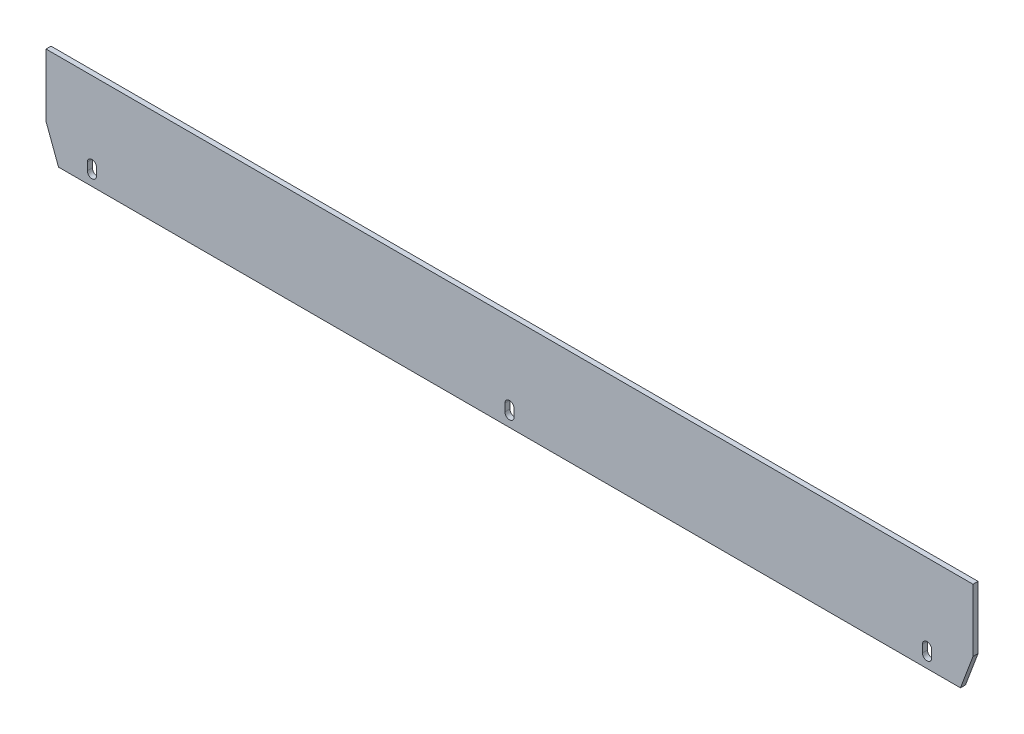
SolidWorks part; units mm, degrees
material "1023 碳钢板 (SS)"
ref_plane "Front Plane" through (0, 0, 0) normal (0, 0, 1) x (1, 0, 0)
ref_plane "Top Plane" through (0, 0, 0) normal (0, 1, 0) x (1, 0, 0)
ref_plane "Right Plane" through (0, 0, 0) normal (1, 0, 0) x (0, 0, -1)
sketch "Sketch1" plane through (0, 0, 0) normal (0, 0, 1) x (1, 0, 0)
  line L1 (555, -57.5) -> (-555, -57.5)
  line L2 (555, -57.5) -> (555, 57.5)
  line L3 (555, 57.5) -> (-555, 57.5)
  line L4 (-555, -57.5) -> (-555, 57.5)
  line L5 (555, -57.5) -> (-555, 57.5) construction
  line L6 (555, 57.5) -> (-555, -57.5) construction
  point P0 (0, 0)
  dimension "D1" = 1110
  dimension "D2" = 115
extrude "Boss-Extrude1" add sketch "Sketch1" along normal blind 6
sketch "Sketch2" plane through (0, 0, 6) normal (0, 0, 1) x (1, 0, 0)
  line L0 (-500, -35) -> (-500, -44) construction
  line L1 (-494.5, -35) -> (-494.5, -44)
  line L2 (-505.5, -35) -> (-505.5, -44)
  line L3 (0, -35) -> (0, -44) construction
  line L4 (5.5, -35) -> (5.5, -44)
  line L5 (-5.5, -35) -> (-5.5, -44)
  line L6 (500, -44) -> (500, -35) construction
  line L7 (494.5, -44) -> (494.5, -35)
  line L8 (505.5, -44) -> (505.5, -35)
  line L9 (-555, -57.5) -> (555, -57.5) construction
  line L10 (-555, -17.5) -> (-540, -57.5)
  line L11 (-555, 57.5) -> (-555, -57.5) construction
  line L12 (-540, -57.5) -> (-555, -57.5)
  line L13 (-555, -57.5) -> (-555, -17.5)
  line L14 (555, -17.5) -> (540, -57.5)
  line L15 (555, -57.5) -> (555, 57.5) construction
  line L16 (540, -57.5) -> (555, -57.5)
  line L17 (555, -57.5) -> (555, -17.5)
  arc A0 (-494.5, -35) -> (-505.5, -35) centre (-500, -35) ccw
  arc A1 (-505.5, -44) -> (-494.5, -44) centre (-500, -44) ccw
  arc A2 (5.5, -35) -> (-5.5, -35) centre (0, -35) ccw
  arc A3 (-5.5, -44) -> (5.5, -44) centre (0, -44) ccw
  arc A4 (494.5, -44) -> (505.5, -44) centre (500, -44) ccw
  arc A5 (505.5, -35) -> (494.5, -35) centre (500, -35) ccw
  point P2 (-500, -39.5)
  point P7 (0, -39.5)
  point P14 (500, -39.5)
  dimension "D1" = 5.5
  dimension "D2" = 9
  dimension "D3" = 500
  dimension "D4" = 500
  dimension "D5" = 18
  dimension "D6" = 40
  dimension "D7" = 15
  dimension "D8" = 40
  dimension "D9" = 15
extrude "Cut-Extrude1" cut sketch "Sketch2" against normal blind 6
